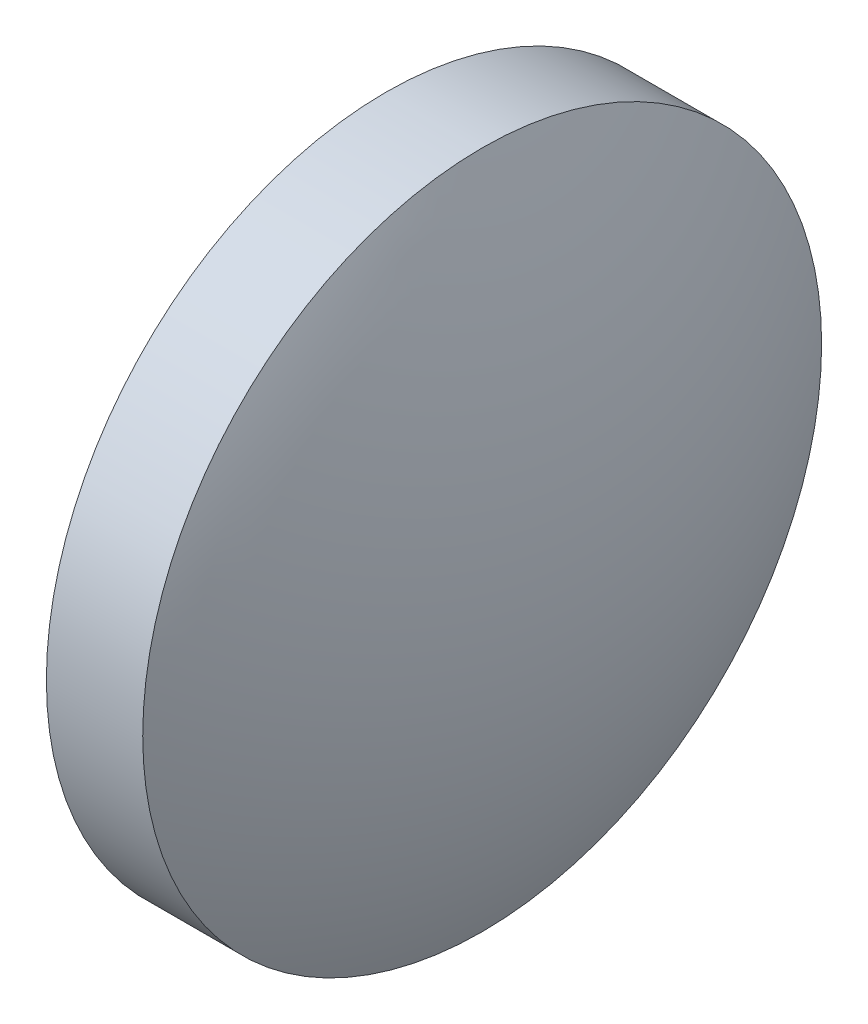
from build123d import *


with BuildPart() as part:
    # Sketch1 → Revolve4 (revolve)
    with BuildSketch(Plane.XY):
        with BuildLine():
            Line((14.64, 0), (9.94, 0))
            ThreePointArc((9.94, 0), (10.306801284, 3.256593068), (11.38882492, 6.35))
            Line((11.38882492, 6.35), (13.19117508, 6.35))
            ThreePointArc((13.19117508, 6.35), (14.273198716, 3.256593068), (14.64, 0))
        make_face()
    revolve(axis=Axis((14.64, 0, 0), (-1, 0, 0)))


solid = part.part
